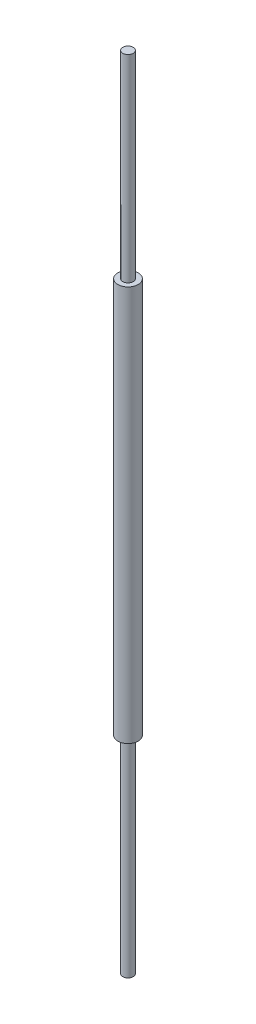
SolidWorks part; units mm, degrees
ref_plane "Front Plane" through (0, 0, 0) normal (0, 0, 1) x (1, 0, 0)
ref_plane "Top Plane" through (0, 0, 0) normal (0, 1, 0) x (1, 0, 0)
ref_plane "Right Plane" through (0, 0, 0) normal (1, 0, 0) x (0, 0, -1)
sketch "Sketch1" plane through (0, 0, 0) normal (1, 0, 0) x (0, 0, -1)
  line L0 (0.45, 16) -> (0.875, 16)
  line L1 (0, -1.75) -> (0.45, -1.75)
  line L2 (0.875, 16) -> (0.875, 50)
  line L3 (0.45, -1.75) -> (0.45, 16)
  line L4 (0.875, 50) -> (0.45, 50)
  line L5 (0.45, 50) -> (0.45, 67)
  line L6 (0.45, 67) -> (0, 67)
  line L7 (0, 67) -> (0, -1.75)
  line L8 (0, -4.3791) -> (0, 69.9257) construction
  line L9 (-3.3, 50.25) -> (3.3, 50.25) construction
  dimension "D1" = 0.45
  dimension "D2" = 52
  dimension "D3" = 0.875
  dimension "D4" = 34
  dimension "D5" = 17
revolve "Revolve1" add sketch "Sketch1" angle 360 about L8
